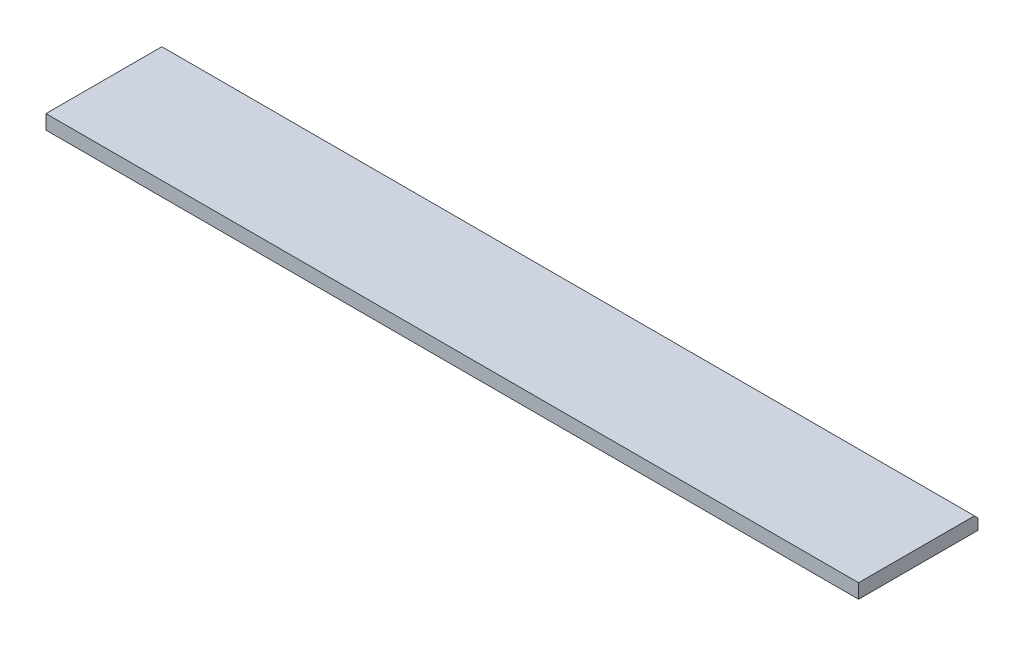
from build123d import *

# Parameters (mm, degrees)
SKETCH_1_W      = 2266
SKETCH_1_H      = 333
EXTRUDE_1_DEPTH = 40
CHAMFER_1_SIZE  = 10


with BuildPart() as part:
    # 草图1 → 凸台-拉伸1 (new body)
    with BuildSketch(Plane(origin=(0, 0, 0), x_dir=(1, 0, 0), z_dir=(0, 1, 0))):
        Rectangle(SKETCH_1_W, SKETCH_1_H)
    extrude(amount=EXTRUDE_1_DEPTH)

    # 倒角1
    chamfer_1_edges = [part.edges().sort_by_distance(p)[0] for p in [
        (0, 40, -166.5),
    ]]
    chamfer(chamfer_1_edges, length=CHAMFER_1_SIZE)


solid = part.part
